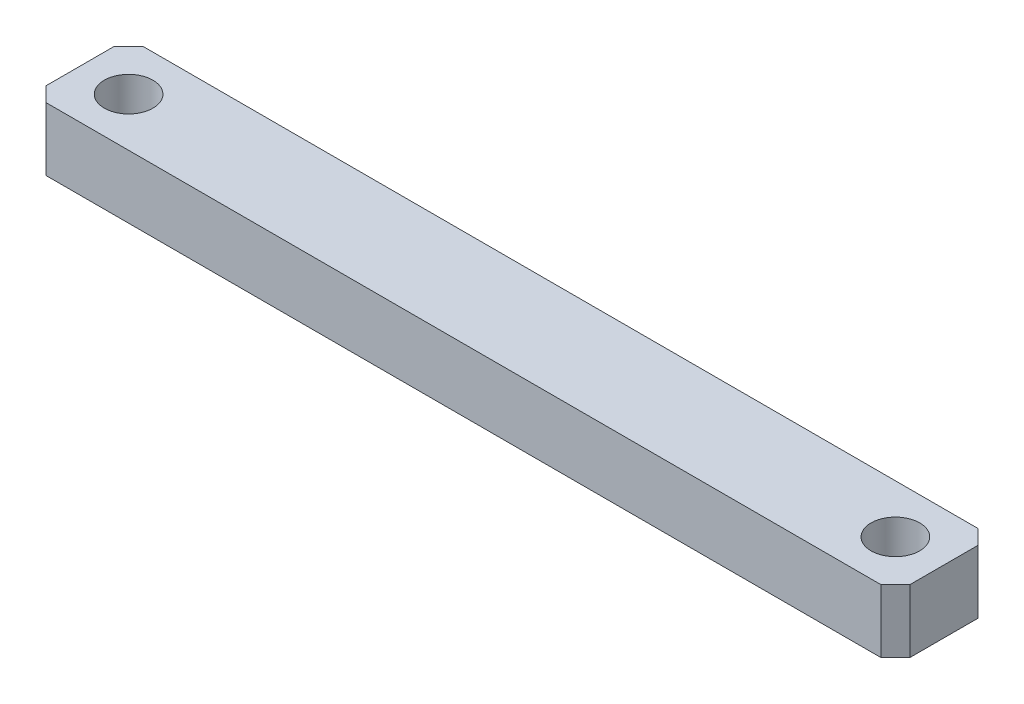
from build123d import *

# Parameters (mm, degrees)
SKETCH1_W           = 177.8
SKETCH1_H           = 13
BOSS_EXTRUDE1_DEPTH = 20
CHAMFER1_SIZE       = 3
SKETCH2_R           = 5
CUT_EXTRUDE1_DEPTH  = 13
LPATTERN1_COUNT     = 2
LPATTERN1_PITCH     = 157.8


with BuildPart() as part:
    # Sketch1 → Boss-Extrude1 (new body)
    with BuildSketch(Plane.XY):
        Rectangle(SKETCH1_W, SKETCH1_H)
    extrude(amount=BOSS_EXTRUDE1_DEPTH)

    # Chamfer1
    chamfer1_edges = [part.edges().sort_by_distance(p)[0] for p in [
        (-88.9, 0, 20),
        (88.9, 0, 20),
        (-88.9, 0, 0),
        (88.9, 0, 0),
    ]]
    chamfer(chamfer1_edges, length=CHAMFER1_SIZE)

    # Sketch2 → Cut-Extrude1 (cut)
    with BuildSketch(Plane(origin=(0, 6.5, 0), x_dir=(1, 0, 0), z_dir=(0, 1, 0))):
        with Locations(Location((-78.9, -10, 0), (0, 0, 180))):
            Circle(SKETCH2_R)
    cut_extrude1 = extrude(amount=-CUT_EXTRUDE1_DEPTH, mode=Mode.SUBTRACT)

    # LPattern1: Cut-Extrude1 ×2
    with Locations(*[(i * LPATTERN1_PITCH, 0, 0) for i in range(1, LPATTERN1_COUNT)]):
        add(cut_extrude1, mode=Mode.SUBTRACT)


solid = part.part
